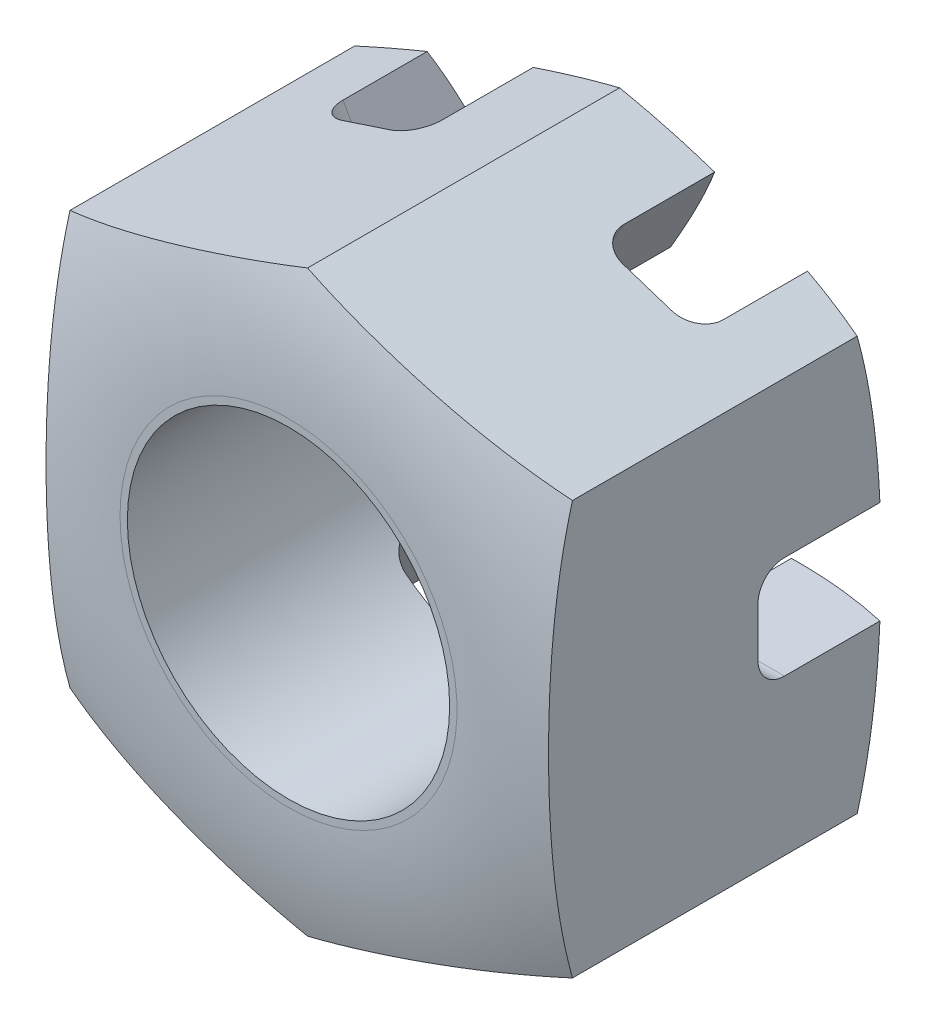
SolidWorks part; units mm, degrees
material "普通碳钢"
ref_plane "Front Plane" through (0, 0, 0) normal (0, 0, 1) x (1, 0, 0)
ref_plane "Top Plane" through (0, 0, 0) normal (0, 1, 0) x (1, 0, 0)
ref_plane "Right Plane" through (0, 0, 0) normal (1, 0, 0) x (0, 0, -1)
sketch "Sketch1" plane through (0, 0, 0) normal (0, 0, 1) x (1, 0, 0)
  line L0 (-103.5007, 0) -> (120.4894, 0) construction
  line L1 (0, 58.0231) -> (0, -56.7163) construction
  line L2 (0, 19.75) -> (-17.15, 14.1137)
  line L3 (-17.15, 14.1137) -> (-17.15, -14.1137)
  line L6 (17.15, -14.1137) -> (17.15, 14.1137)
  line L7 (17.15, 14.1137) -> (0, 19.75)
  line L8 (-17.15, -14.1137) -> (0, -19.75)
  line L9 (0, -19.75) -> (17.15, -14.1137)
  dimension "D1" = 34.3
  dimension "D2" = 39.5
extrude "Boss-Extrude1" add sketch "Sketch1" along normal blind 23.9
sketch "Sketch3" plane through (0, 0, 0) normal (0, 0, -1) x (-1, 0, 0)
  line L0 (-32.5, 3.5) -> (32.5, 3.5)
  line L1 (32.5, 3.5) -> (32.5, -3.5)
  line L2 (-32.5, -3.5) -> (32.5, -3.5)
  line L3 (-32.5, -3.5) -> (-32.5, 3.5)
  line L4 (55, 0) -> (-55, 0) construction
  line L5 (0, 55) -> (0, -55) construction
  dimension "D1" = 65
  dimension "D2" = 3.5
  dimension "D3" = 7
  dimension "D4" = 32.5
extrude "Cut-Extrude1" cut sketch "Sketch3" against normal blind 9
ref_axis "Axis1" through (0, 0, -1.73) along (0, 0, 1)
pattern_circular "CirPattern1" count 3 over 120 about axis through (0, 0, 0) along (0, 0, 1) of "Cut-Extrude1"
hole_wizard "M24x2.0 Tapped Hole1" positions "Sketch7" profile "Sketch6" tap size "M24x2.0" standard "GB" end condition through all
sketch "Sketch7" plane through (0, 0, 23.9) normal (0, 0, 1) x (1, 0, 0)
  point P0 (0, 0)
sketch "Sketch6" plane through (0, 0, 23.9) normal (1, 0, 0) x (0, -1, 0)
  line L0 (0, 0) -> (0, 23.9)
  line L1 (0, 23.9) -> (11, 23.9)
  line L2 (11, 23.9) -> (11, 0)
  line L5 (11, 0) -> (0, 0)
  line L11 (0, -6.35) -> (0, 107.95) construction
  dimension "通孔螺纹孔钻头直径" = 22
  dimension "通孔螺纹孔钻头深度" = 23.9
cosmetic thread "CosmeticThread Hole thread1" parameters "D2"=24
fillet "Fillet2" radius 1.8 12 edges at (-10.6132, -11.3825, 9) (-4.1852, -14.2489, 9) (4.1852, -14.2489, 9) (10.6132, -11.3825, 9) (13.7892, -3.5, 9) (13.7892, 3.5, 9) (10.6132, 11.3825, 9) (4.1852, 14.2489, 9) (-4.1852, 14.2489, 9) (-10.6132, 11.3825, 9) (-13.7892, 3.5, 9) (-13.7892, -3.5, 9)
sketch "Sketch8" plane through (0, 0, 0) normal (0, 1, 0) x (1, 0, 0)
  line L0 (0, -13.145) -> (0, 13.145) construction
  line L1 (17.15, 0) -> (12.981, 0) construction
  line L2 (17.15, -23.9) -> (0, -23.9) construction
  line L3 (11.5, 0) -> (33.5205, 0)
  line L4 (33.5205, 0) -> (33.5205, -11.5246)
  line L6 (11.5, -23.9) -> (28.8302, -23.9)
  line L7 (28.8302, -23.9) -> (28.8302, -17.5427)
  arc A0 (11.5, -23.9) -> (28.8302, -17.5427) centre (11.5, 2.9) ccw
  arc A1 (33.5205, -11.5246) -> (11.5, 0) centre (11.5, -26.8) ccw
  dimension "D1" = 53.6
  dimension "D4" = 11.5
  dimension "D6" = 53.6
  dimension "D2" = 11.5
  dimension "D3" = 26.8
  dimension "D5" = 26.8
revolve "Cut-Revolve1" cut sketch "Sketch8" angle 360 about axis through (0, 0, -1.73) along (0, 0, 1)
